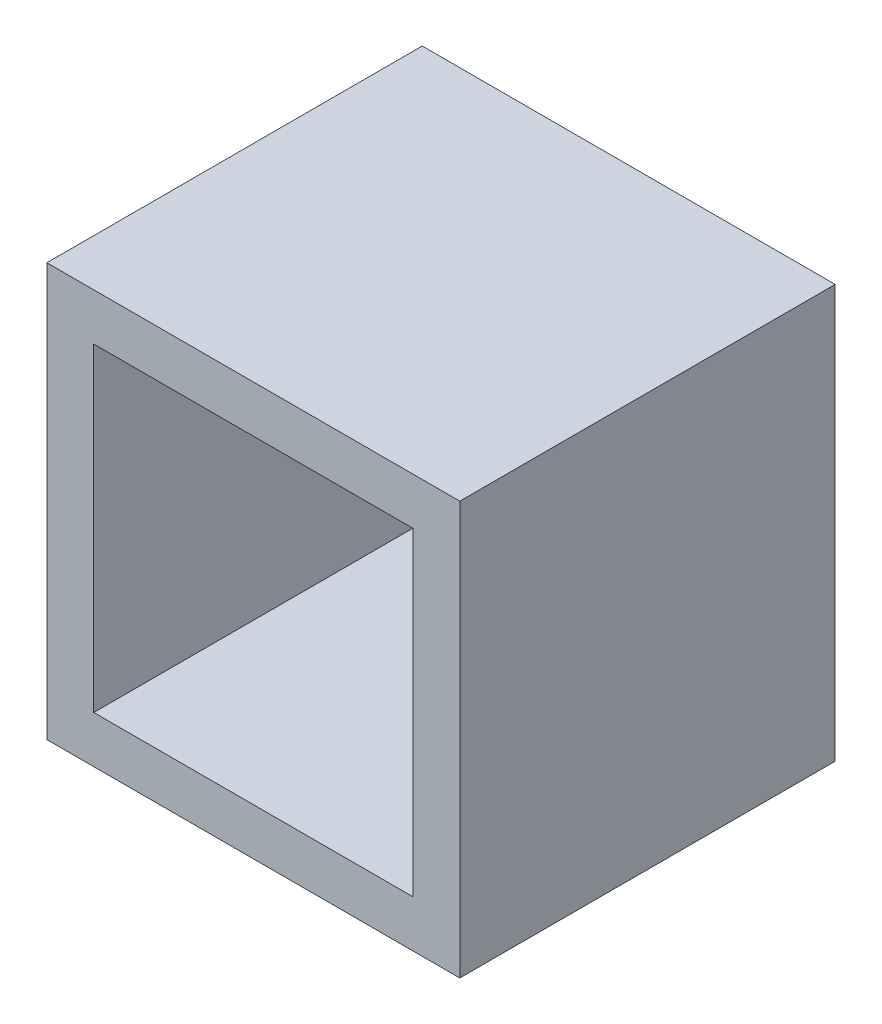
from build123d import *

# Parameters (mm, degrees)
SKETCH_1_W      = 66
SKETCH_1_H      = 66
SKETCH_1_W_2    = 51
SKETCH_1_H_2    = 51
EXTRUDE_1_DEPTH = 30


with BuildPart() as part:
    # 草图1 → 凸台-拉伸1 (new, symmetric)
    with BuildSketch(Plane.XY):
        Rectangle(SKETCH_1_W, SKETCH_1_H)
        Rectangle(SKETCH_1_W_2, SKETCH_1_H_2, mode=Mode.SUBTRACT)
    extrude(amount=EXTRUDE_1_DEPTH, both=True)


solid = part.part
